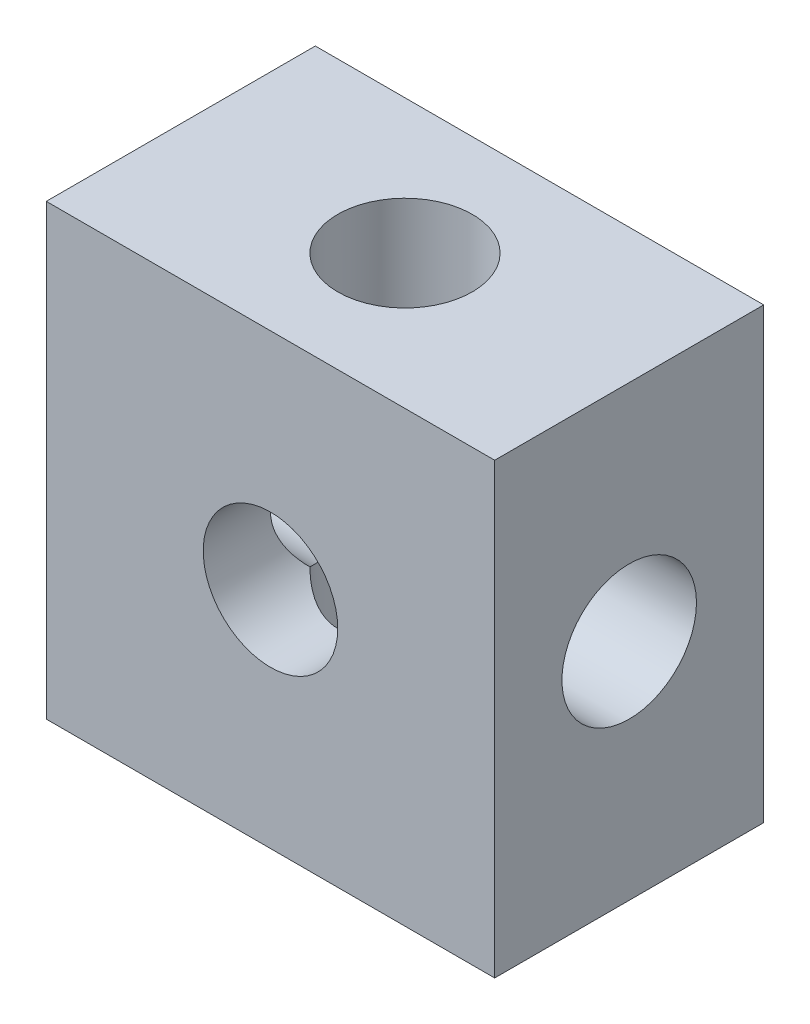
from build123d import *

# Parameters (mm, degrees)
SKETCH_1_W          = 10
SKETCH_1_H          = 6
EXTRUDE_1_DEPTH     = 10
SKETCH_2_R          = 1.5
CUT_EXTRUDE_1_DEPTH = 16.362291496
SKETCH_4_R          = 1.5
CUT_EXTRUDE_2_DEPTH = 16.362291496
SKETCH_3_R          = 1.5
CUT_EXTRUDE_3_DEPTH = 16.362291496


with BuildPart() as part:
    # 草图1 → 凸台-拉伸1 (new body)
    with BuildSketch(Plane(origin=(0, 0, 0), x_dir=(1, 0, 0), z_dir=(0, 1, 0))):
        with Locations((5, 3)):
            Rectangle(SKETCH_1_W, SKETCH_1_H)
    extrude(amount=EXTRUDE_1_DEPTH)

    # 草图2 → 切除-拉伸1 (cut, through all)
    with BuildSketch(Plane.XY):
        with Locations((5, 5)):
            Circle(SKETCH_2_R)
    extrude(amount=-CUT_EXTRUDE_1_DEPTH, mode=Mode.SUBTRACT)

    # 草图4 → 切除-拉伸2 (cut, through all)
    with BuildSketch(Plane(origin=(0, 10, 0), x_dir=(1, 0, 0), z_dir=(0, 1, 0))):
        with Locations(Location((5, 3, 0), (0, 0, 270))):
            Circle(SKETCH_4_R)
    extrude(amount=-CUT_EXTRUDE_2_DEPTH, mode=Mode.SUBTRACT)

    # 草图3 → 切除-拉伸3 (cut, through all)
    with BuildSketch(Plane(origin=(10, 0, 0), x_dir=(0, 0, -1), z_dir=(1, 0, 0))):
        with Locations((3, 5)):
            Circle(SKETCH_3_R)
    extrude(amount=-CUT_EXTRUDE_3_DEPTH, mode=Mode.SUBTRACT)


solid = part.part
